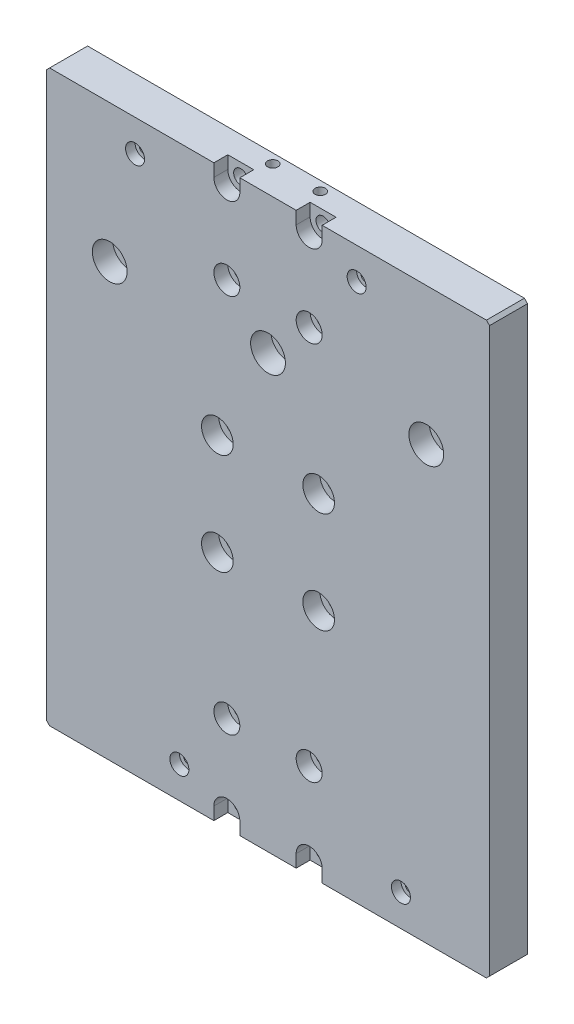
SolidWorks part; units mm, degrees
material "AL7075"
ref_plane "Front Plane" through (0, 0, 0) normal (0, 0, 1) x (1, 0, 0)
ref_plane "Top Plane" through (0, 0, 0) normal (0, 1, 0) x (1, 0, 0)
ref_plane "Right Plane" through (0, 0, 0) normal (1, 0, 0) x (0, 0, -1)
sketch "Sketch1" plane through (0, 0, 0) normal (0, 0, 1) x (1, 0, 0)
  line L1 (-70, 90) -> (70, 90)
  line L2 (-70, 90) -> (-70, -90)
  line L3 (-70, -90) -> (70, -90)
  line L4 (70, 90) -> (70, -90)
  line L5 (-70, 90) -> (70, -90) construction
  line L6 (-70, -90) -> (70, 90) construction
  point P0 (0, 0)
  dimension "D1" = 140
  dimension "D2" = 180
extrude "Boss-Extrude1" add sketch "Sketch1" along normal mid plane 12
hole_wizard "CBORE for M4 Hex Socket Head Cap Screw2" positions "Sketch4" profile "Sketch5" counterbore size "M4" standard "ISO" end condition through all
sketch "Sketch4" plane through (0, 0, 6) normal (0, 0, 1) x (1, 0, 0)
  point P0 (13, -60)
  point P3 (-13, -60)
  point P6 (-13, -86)
  point P9 (13, -86)
  point P12 (-13, 86)
  point P15 (13, 86)
  point P18 (-13, 60)
  point P21 (13, 60)
sketch "Sketch5" plane through (13, -60, 6) normal (1, 0, 0) x (0, -1, 0)
  line L0 (0, 0) -> (0, 12)
  line L1 (0, 12) -> (2.25, 12)
  line L3 (2.25, 12) -> (2.25, 4.4)
  line L4 (2.25, 4.4) -> (4.1, 4.4)
  line L5 (4.1, 4.4) -> (4.1, 0)
  line L7 (4.1, 0) -> (0, 0)
  line L11 (0, -6.35) -> (0, 107.95) construction
  dimension "通孔孔直径" = 4.5
  dimension "通孔孔深度" = 12
  dimension "柱形沉头孔直径" = 8.2
  dimension "柱形沉头孔深度" = 4.4
hole_wizard "Size mm dowel hole 1" positions "Sketch6" profile "Sketch7" hole size "Ø5.0" standard "ISO"
sketch "Sketch6" plane through (0, 0, -6) normal (0, 0, -1) x (-1, 0, 0)
  line L0 (19.7, 56) -> (-19.7, 56) construction
  line L1 (-19.7, 88.2428) -> (-19.7, 57.8428) construction
  line L2 (19.7, 64) -> (19.7, 57) construction
  line L3 (19.7, -56) -> (-19.7, -56) construction
  point P2 (14.7, -51)
  point P4 (-14.7, -51)
  point P6 (14.7, 53.5)
  point P8 (-14.7, 53.5)
  dimension "D1" = 2.5
  dimension "D2" = 5
  dimension "D3" = 5
  dimension "D4" = 5
sketch "Sketch7" plane through (-14.7, -51, -6) normal (1, 0, 0) x (0, 1, 0)
  line L0 (0, 0) -> (0, 11.5022)
  line L1 (0, 11.5022) -> (2.5, 10)
  line L2 (2.5, 10) -> (2.5, 0)
  line L5 (2.5, 0) -> (0, 0)
  line L10 (0, 11.5022) -> (-2.5, 10) construction
  line L11 (0, -6.35) -> (0, 107.95) construction
  dimension "孔直径" = 5
  dimension "孔深度" = 10
  dimension "导头角度" = 118
hole_wizard "CBORE for M5 Hex Socket Head Cap Screw1" positions "Sketch8" profile "Sketch9" counterbore size "M5" standard "ISO" end condition through all
sketch "Sketch8" plane through (0, 0, 6) normal (0, 0, 1) x (1, 0, 0)
  point P0 (16, 16)
  point P3 (-16, 16)
  point P6 (-16, -16)
  point P9 (16, -16)
sketch "Sketch9" plane through (16, 16, 6) normal (1, 0, 0) x (0, -1, 0)
  line L0 (0, 0) -> (0, 12)
  line L1 (0, 12) -> (2.75, 12)
  line L3 (2.75, 12) -> (2.75, 5.4)
  line L4 (2.75, 5.4) -> (5, 5.4)
  line L5 (5, 5.4) -> (5, 0)
  line L7 (5, 0) -> (0, 0)
  line L11 (0, -6.35) -> (0, 107.95) construction
  dimension "通孔孔直径" = 5.5
  dimension "通孔孔深度" = 12
  dimension "柱形沉头孔直径" = 10
  dimension "柱形沉头孔深度" = 5.4
sketch "Sketch10" plane through (0, 0, 6) normal (0, 0, 1) x (1, 0, 0)
  line L0 (0, 0) -> (103.8849, 0) construction
  line L1 (-17.1, 90) -> (-8.9, 90)
  line L2 (-17.1, 90) -> (-17.1, 86)
  line L3 (-17.1, 86) -> (-8.9, 86)
  line L4 (-8.9, 90) -> (-8.9, 86)
  line L5 (-17.1, 90) -> (-8.9, 86) construction
  line L6 (-17.1, 86) -> (-8.9, 90) construction
  line L7 (8.9, 90) -> (17.1, 90)
  line L8 (8.9, 90) -> (8.9, 86)
  line L9 (8.9, 86) -> (17.1, 86)
  line L10 (17.1, 90) -> (17.1, 86)
  line L11 (8.9, 90) -> (17.1, 86) construction
  line L12 (8.9, 86) -> (17.1, 90) construction
  line L13 (12.1, 90) -> (-12.1, 90) construction
  line L14 (-12.1, -90) -> (12.1, -90) construction
  line L15 (-17.1, -86) -> (-8.9, -86)
  line L16 (-17.1, -86) -> (-17.1, -90)
  line L17 (-17.1, -90) -> (-8.9, -90)
  line L18 (-8.9, -86) -> (-8.9, -90)
  line L19 (-17.1, -86) -> (-8.9, -90) construction
  line L20 (-17.1, -90) -> (-8.9, -86) construction
  line L21 (8.9, -86) -> (17.1, -86)
  line L22 (8.9, -86) -> (8.9, -90)
  line L23 (8.9, -90) -> (17.1, -90)
  line L24 (17.1, -86) -> (17.1, -90)
  line L25 (8.9, -86) -> (17.1, -90) construction
  line L26 (8.9, -90) -> (17.1, -86) construction
  arc A2 (-12.1, -90) -> (-13.9, -90) centre (-13, -86) ccw construction
  arc A3 (13.9, -90) -> (12.1, -90) centre (13, -86) ccw construction
  arc A4 (12.1, 90) -> (13.9, 90) centre (13, 86) ccw construction
  arc A5 (-13.9, 90) -> (-12.1, 90) centre (-13, 86) ccw construction
  point P0 (-13, 88)
  point P5 (13, 88)
  point P13 (13, -88)
  point P23 (-13, -88)
extrude "Cut-Extrude1" cut sketch "Sketch10" against normal up to surface (4.4 mm away) up to face at (-10.75, -86, 1.6)
hole_wizard "M4 Tapped Hole1" positions "Sketch11" profile "Sketch12" tap size "M4" standard "ISO"
sketch "Sketch11" plane through (0, 90, 0) normal (0, 1, 0) x (1, 0, 0)
  line L0 (-5, 1) -> (-5, 5) construction
  line L2 (10, 1) -> (10, 5) construction
  arc A0 (-10, 1) -> (-5, 1) centre (-7.5, 1) ccw construction
  point P0 (-7.5, 3)
  point P2 (7.5, 3)
  dimension "D1" = 2.5
  dimension "D2" = 2
  dimension "D3" = 2.5
sketch "Sketch12" plane through (-7.5, 90, -3) normal (1, 0, 0) x (0, 0, 1)
  line L0 (0, 0) -> (0, 16.4914)
  line L1 (0, 16.4914) -> (1.65, 15.5)
  line L2 (1.65, 15.5) -> (1.65, 0)
  line L5 (1.65, 0) -> (0, 0)
  line L10 (0, 16.4914) -> (-1.65, 15.5) construction
  line L11 (0, -6.35) -> (0, 107.95) construction
  dimension "螺纹孔钻头直径" = 3.3
  dimension "螺纹孔钻头深度" = 15.5
  dimension "导头角度" = 118
cosmetic thread "Cosmetic thread 1" parameters "D1"=12, "D2"=4
cosmetic thread "Cosmetic thread 2" parameters "D1"=12, "D2"=4
hole_wizard "Size mm dowel hole 2" positions "Sketch13" profile "Sketch14" hole size "Ø6.0" standard "ISO"
sketch "Sketch13" plane through (0, 0, 6) normal (0, 0, 1) x (1, 0, 0)
  point P0 (28, 80)
  point P3 (-42, 80)
  point P6 (42, -80)
  point P9 (-28, -80)
sketch "Sketch14" plane through (28, 80, 6) normal (1, 0, 0) x (0, -1, 0)
  line L0 (0, 0) -> (0, 3)
  line L1 (0, 3) -> (3, 3)
  line L2 (3, 3) -> (3, 0)
  line L5 (3, 0) -> (0, 0)
  line L10 (0, 3) -> (-3, 3) construction
  line L11 (0, -6.35) -> (0, 107.95) construction
  dimension "孔直径" = 6
  dimension "孔深度" = 3
  dimension "导头角度" = 180
hole_wizard "CBORE for M3 Hex Socket Head Cap Screw1" positions "Sketch15" profile "Sketch16" counterbore size "M3" standard "ISO" end condition through all
sketch "Sketch15" plane through (0, 0, -6) normal (0, 0, -1) x (-1, 0, 0)
  point P2 (-28, 80)
  point P5 (42, 80)
  point P8 (28, -80)
  point P11 (-42, -80)
sketch "Sketch16" plane through (28, 80, -6) normal (1, 0, 0) x (0, 1, 0)
  line L0 (0, 0) -> (0, 12)
  line L1 (0, 12) -> (1.7, 12)
  line L3 (1.7, 12) -> (1.7, 3.4)
  line L4 (1.7, 3.4) -> (3.25, 3.4)
  line L5 (3.25, 3.4) -> (3.25, 0)
  line L7 (3.25, 0) -> (0, 0)
  line L11 (0, -6.35) -> (0, 107.95) construction
  dimension "通孔孔直径" = 3.4
  dimension "通孔孔深度" = 12
  dimension "柱形沉头孔直径" = 6.5
  dimension "柱形沉头孔深度" = 3.4
chamfer "Chamfer1" distance 1 angle 45 4 edges at (70, 90, 0) (70, -90, 0) (-70, -90, 0) (-70, 90, 0)
hole_wizard "CBORE for M6 Hex Socket Head Cap Screw1" positions "Sketch17" profile "Sketch18" counterbore size "M6" standard "ISO" end condition through all
sketch "Sketch17" plane through (0, 0, 6) normal (0, 0, 1) x (1, 0, 0)
  line L0 (-70, 46.5) -> (70, 46.5) construction
  line L1 (-70, 89) -> (-70, -89) construction
  line L2 (70, -89) -> (70, 89) construction
  line L5 (69, 90) -> (17.1, 90) construction
  line L6 (0, -90) -> (0, 90) construction
  line L7 (-8.9, -90) -> (8.9, -90) construction
  line L8 (8.9, 90) -> (-8.9, 90) construction
  point P24 (0, 46.5)
  point P26 (50, 46.5)
  point P29 (-50, 46.5)
  dimension "D1" = 43.5
  dimension "D2" = 100
sketch "Sketch18" plane through (-50, 46.5, 6) normal (1, 0, 0) x (0, -1, 0)
  line L0 (0, 0) -> (0, 12)
  line L1 (0, 12) -> (3.3, 12)
  line L3 (3.3, 12) -> (3.3, 6.4)
  line L4 (3.3, 6.4) -> (5.5, 6.4)
  line L5 (5.5, 6.4) -> (5.5, 0)
  line L7 (5.5, 0) -> (0, 0)
  line L11 (0, -6.35) -> (0, 107.95) construction
  dimension "通孔孔直径" = 6.6
  dimension "通孔孔深度" = 12
  dimension "柱形沉头孔直径" = 11
  dimension "柱形沉头孔深度" = 6.4
